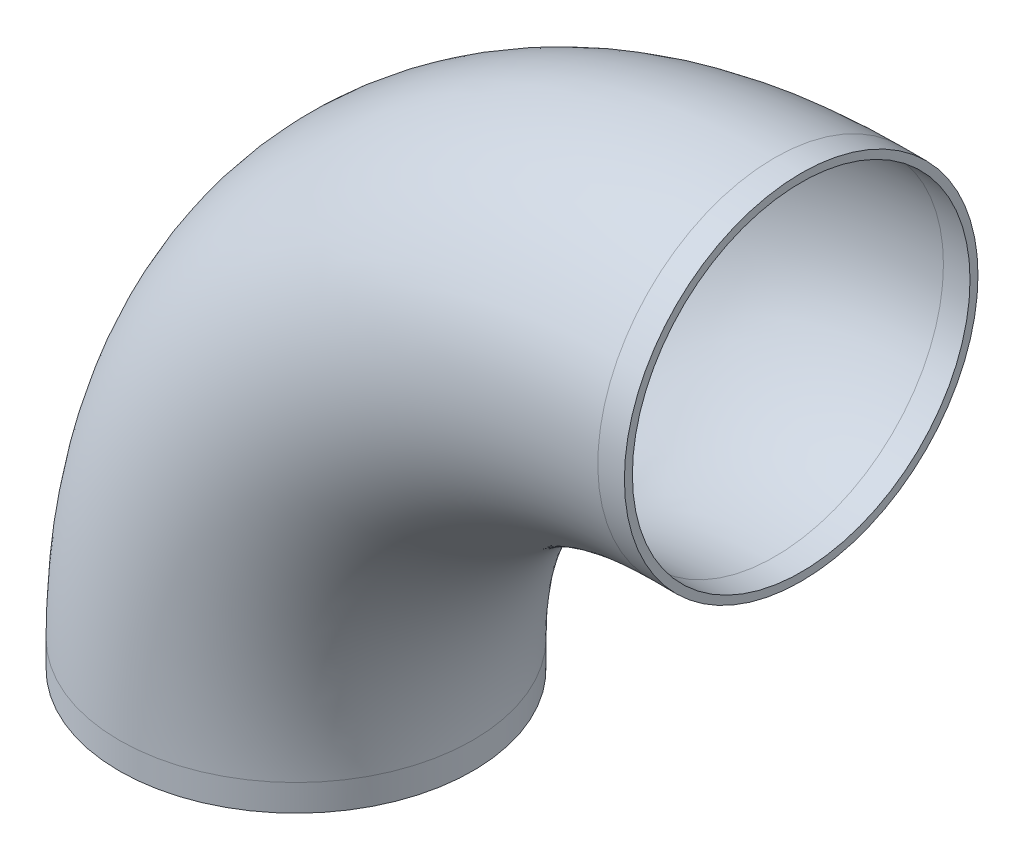
SolidWorks part; units mm, degrees
material "304不锈钢  "
ref_plane "Front Plane" through (0, 0, 0) normal (0, 0, 1) x (1, 0, 0)
ref_plane "Top Plane" through (0, 0, 0) normal (0, 1, 0) x (1, 0, 0)
ref_plane "Right Plane" through (0, 0, 0) normal (1, 0, 0) x (0, 0, -1)
sketch "Sketch1" plane through (0, 0, 0) normal (0, 1, 0) x (1, 0, 0)
  circle A0 centre (0, 0) radius 66.5
  dimension "D2" = 133
sketch3d "3DSketch1"
  circle A1 centre (0, 0, 0) radius 66.5
  circle A3 centre (0, 0, 0) radius 66.5
  circle A4 centre (0, 0, 0) radius 66.5
  circle A5 centre (0, 0, 0) radius 66.5
  point P5 (0, 66.5, 0)
  point P7 (0, 66.5, 0)
  point P10 (0, 66.5, 0)
  point P12 (0, 66.5, 0)
  dimension "D1" = 0
  dimension "D2" = 0
sketch "Sketch2" plane through (0, 0, 0) normal (0, 0, 1) x (1, 0, 0)
  line L2 (0, 0) -> (0, 10)
  line L3 (180, 190) -> (190, 190)
  arc A0 (0, 10) -> (180, 190) centre (180, 10) cw
  point P8 (0, 190)
  dimension "D3" = 180
  dimension "D1" = 190
  dimension "D2" = 190
sweep "Sweep1" add profiles "Sketch1" path "Sketch2"
shell "Shell1" thickness 3
